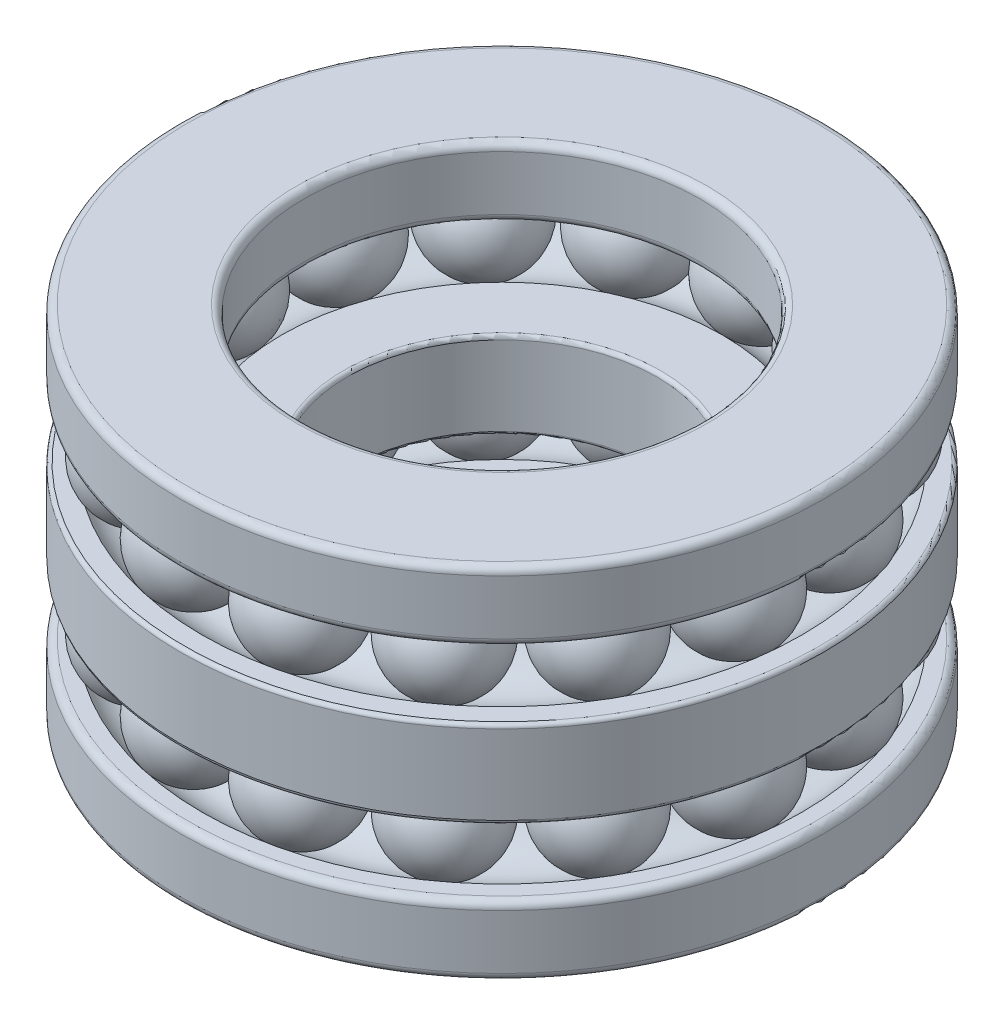
SolidWorks part; units mm, degrees
ref_plane "Front Plane" through (0, 0, 0) normal (0, 0, 1) x (1, 0, 0)
ref_plane "Top Plane" through (0, 0, 0) normal (0, 1, 0) x (1, 0, 0)
ref_plane "Right Plane" through (0, 0, 0) normal (1, 0, 0) x (0, 0, -1)
sketch "Sketch1" plane through (0, 0, 0) normal (1, 0, 0) x (0, 0, -1)
  line L0 (0, 45.3274) -> (0, 0) construction
  line L1 (0, 0) -> (72.1692, 0) construction
  line L2 (21, 8.9) -> (21, 8.6) construction
  line L3 (12.8, 3.5) -> (25.7, 3.5)
  line L4 (12.5, 3.2) -> (12.5, -3.2)
  line L5 (12.8, -3.5) -> (25.7, -3.5)
  line L6 (26, 3.2) -> (26, -3.2)
  line L7 (16.6, 14.5) -> (25.4, 14.5)
  line L8 (16, 13.9) -> (16, 9.5)
  line L9 (16.6, 8.9) -> (25.4, 8.9)
  line L10 (26, 13.9) -> (26, 9.5)
  line L11 (21, 8.6) -> (21, 8) construction
  line L12 (21, 6.2) -> (25.2, 6.2) construction
  line L13 (21, -8.6) -> (21, -8) construction
  line L14 (21, -8.9) -> (21, -8.6) construction
  line L15 (26, -13.9) -> (26, -9.5)
  line L16 (16.6, -8.9) -> (25.4, -8.9)
  line L17 (16, -13.9) -> (16, -9.5)
  line L18 (16.6, -14.5) -> (25.4, -14.5)
  arc A0 (16, 9.5) -> (16.6, 8.9) centre (16.6, 9.5) ccw
  arc A1 (16.6, 14.5) -> (16, 13.9) centre (16.6, 13.9) ccw
  arc A2 (25.4, 8.9) -> (26, 9.5) centre (25.4, 9.5) ccw
  arc A3 (25.4, 14.5) -> (26, 13.9) centre (25.4, 13.9) cw
  arc A4 (25.7, 3.5) -> (26, 3.2) centre (25.7, 3.2) cw
  arc A5 (25.7, -3.5) -> (26, -3.2) centre (25.7, -3.2) ccw
  arc A6 (12.5, -3.2) -> (12.8, -3.5) centre (12.8, -3.2) ccw
  arc A7 (12.8, 3.5) -> (12.5, 3.2) centre (12.8, 3.2) ccw
  circle A8 centre (21, 6.2) radius 4.2
  circle A9 centre (21, -6.2) radius 4.2
  arc A10 (25.4, -14.5) -> (26, -13.9) centre (25.4, -13.9) ccw
  arc A11 (25.4, -8.9) -> (26, -9.5) centre (25.4, -9.5) cw
  arc A12 (16.6, -14.5) -> (16, -13.9) centre (16.6, -13.9) cw
  arc A13 (16, -9.5) -> (16.6, -8.9) centre (16.6, -9.5) cw
  point P25 (26, 3.5)
  point P28 (26, -3.5)
  point P35 (21, 14.5)
  dimension "D4" = 0.6
  dimension "D5" = 0.3
  dimension "D7" = 8.4
  dimension "D1" = 32
  dimension "r1" = 0.3
  dimension "r" = 0.6
  dimension "D" = 52
  dimension "d3" = 52
  dimension "d2" = 25
  dimension "B" = 7
  dimension "T1" = 29
  dimension "D6" = 5.6
sketch "Sketch2" plane through (0, 0, 0) normal (1, 0, 0) x (0, 0, -1)
  line L0 (16, 13.9) -> (16, 9.5) construction
  line L1 (16.6, 8.9) -> (25.4, 8.9) construction
  line L2 (26, 13.9) -> (26, 9.5) construction
  line L3 (16.6, 14.5) -> (25.4, 14.5) construction
  line L4 (12.5, 3.2) -> (12.5, -3.2) construction
  line L5 (12.8, -3.5) -> (25.7, -3.5) construction
  line L6 (26, 3.2) -> (26, -3.2) construction
  line L7 (12.8, 3.5) -> (25.7, 3.5) construction
  line L8 (16, -13.9) -> (16, -9.5) construction
  line L9 (16.6, -8.9) -> (25.4, -8.9) construction
  line L10 (26, -13.9) -> (26, -9.5) construction
  line L11 (16.6, -14.5) -> (25.4, -14.5) construction
  line L12 (16, 13.9) -> (16, 9.5)
  line L13 (16.6, 8.9) -> (17.7829, 8.9)
  line L14 (26, 13.9) -> (26, 9.5)
  line L15 (16.6, 14.5) -> (25.4, 14.5)
  line L16 (12.5, 3.2) -> (12.5, -3.2)
  line L17 (12.8, -3.5) -> (17.7829, -3.5)
  line L18 (26, 3.2) -> (26, -3.2)
  line L19 (12.8, 3.5) -> (17.7829, 3.5)
  line L20 (16, -13.9) -> (16, -9.5)
  line L21 (16.6, -8.9) -> (17.7829, -8.9)
  line L22 (26, -13.9) -> (26, -9.5)
  line L23 (16.6, -14.5) -> (25.4, -14.5)
  line L24 (24.2171, 3.5) -> (25.7, 3.5)
  line L25 (24.2171, 8.9) -> (25.4, 8.9)
  line L26 (24.2171, -3.5) -> (25.7, -3.5)
  line L27 (24.2171, -8.9) -> (25.4, -8.9)
  line L28 (0, 0) -> (0, 69.2895) construction
  arc A0 (16, 9.5) -> (16.6, 8.9) centre (16.6, 9.5) ccw construction
  arc A1 (25.4, 8.9) -> (26, 9.5) centre (25.4, 9.5) ccw construction
  arc A2 (26, 13.9) -> (25.4, 14.5) centre (25.4, 13.9) ccw construction
  arc A3 (16.6, 14.5) -> (16, 13.9) centre (16.6, 13.9) ccw construction
  arc A4 (12.5, -3.2) -> (12.8, -3.5) centre (12.8, -3.2) ccw construction
  arc A5 (25.7, -3.5) -> (26, -3.2) centre (25.7, -3.2) ccw construction
  arc A6 (26, 3.2) -> (25.7, 3.5) centre (25.7, 3.2) ccw construction
  arc A7 (12.8, 3.5) -> (12.5, 3.2) centre (12.8, 3.2) ccw construction
  arc A8 (16.6, -8.9) -> (16, -9.5) centre (16.6, -9.5) ccw construction
  arc A9 (26, -9.5) -> (25.4, -8.9) centre (25.4, -9.5) ccw construction
  arc A10 (25.4, -14.5) -> (26, -13.9) centre (25.4, -13.9) ccw construction
  arc A11 (16, -13.9) -> (16.6, -14.5) centre (16.6, -13.9) ccw construction
  circle A12 centre (21, -6.2) radius 4.2 construction
  circle A13 centre (21, 6.2) radius 4.2 construction
  arc A14 (16, 9.5) -> (16.6, 8.9) centre (16.6, 9.5) ccw
  arc A15 (25.4, 8.9) -> (26, 9.5) centre (25.4, 9.5) ccw
  arc A16 (26, 13.9) -> (25.4, 14.5) centre (25.4, 13.9) ccw
  arc A17 (16.6, 14.5) -> (16, 13.9) centre (16.6, 13.9) ccw
  arc A18 (12.5, -3.2) -> (12.8, -3.5) centre (12.8, -3.2) ccw
  arc A19 (25.7, -3.5) -> (26, -3.2) centre (25.7, -3.2) ccw
  arc A20 (26, 3.2) -> (25.7, 3.5) centre (25.7, 3.2) ccw
  arc A21 (12.8, 3.5) -> (12.5, 3.2) centre (12.8, 3.2) ccw
  arc A22 (16.6, -8.9) -> (16, -9.5) centre (16.6, -9.5) ccw
  arc A23 (26, -9.5) -> (25.4, -8.9) centre (25.4, -9.5) ccw
  arc A24 (25.4, -14.5) -> (26, -13.9) centre (25.4, -13.9) ccw
  arc A25 (16, -13.9) -> (16.6, -14.5) centre (16.6, -13.9) ccw
  arc A26 (24.2171, -3.5) -> (17.7829, -3.5) centre (21, -6.2) ccw
  arc A27 (17.7829, 3.5) -> (24.2171, 3.5) centre (21, 6.2) ccw
  arc A28 (24.2171, 8.9) -> (17.7829, 8.9) centre (21, 6.2) ccw
  arc A29 (17.7829, -8.9) -> (24.2171, -8.9) centre (21, -6.2) ccw
revolve "Revolve1" add sketch "Sketch2" angle 360 mid plane about L28
sketch "Sketch3" plane through (0, 0, 0) normal (1, 0, 0) x (0, 0, -1)
  line L0 (21, 10.4) -> (21, -10.4)
  circle A0 centre (21, 6.2) radius 4.2 construction
  circle A1 centre (21, -6.2) radius 4.2 construction
  arc A2 (21, 2) -> (21, 10.4) centre (21, 6.2) ccw
  arc A3 (21, -10.4) -> (21, -2) centre (21, -6.2) ccw
revolve "Revolve2" add sketch "Sketch3" angle 360 mid plane about L0
pattern_circular "CirPattern5" count 15 over 360 about axis through (0, 0, 0) along (0, 1, 0)
